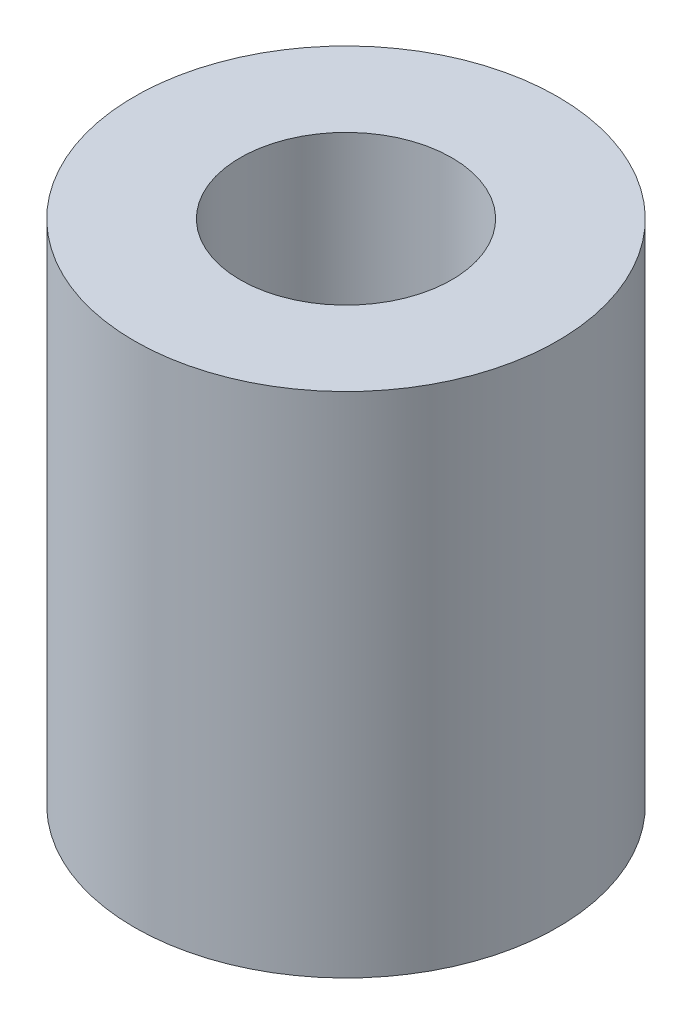
from build123d import *

# Parameters (mm, degrees)
SKETCH_1_R         = 2.5
EXTRUDE_1_DEPTH    = 6
HOLE_WIZARD_M3_1_D = 2.5


with BuildPart() as part:
    # 草图1 → 凸台-拉伸1 (new body)
    with BuildSketch(Plane(origin=(0, 0, 0), x_dir=(1, 0, 0), z_dir=(0, 1, 0))):
        with Locations(Location((0, 0, 0), (0, 0, 270))):
            Circle(SKETCH_1_R)
    extrude(amount=EXTRUDE_1_DEPTH)

    # M3 螺纹孔1 (through all)
    with Locations(Plane(origin=(0, 6, 0), x_dir=(1, 0, 0), z_dir=(0, 1, 0))):
        with Locations((0, 0)):
            Hole(HOLE_WIZARD_M3_1_D / 2)


solid = part.part
